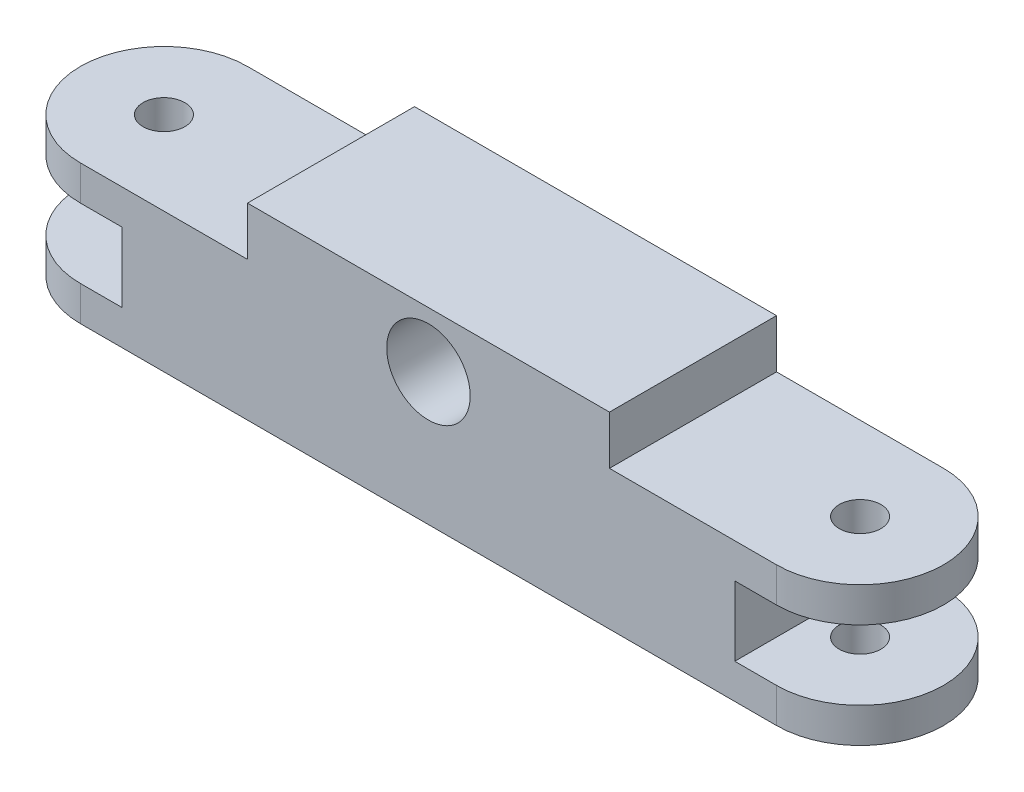
SolidWorks part; units mm, degrees
material "Plain carbon steel"
ref_plane "Front Plane" through (0, 0, 0) normal (0, 0, 1) x (1, 0, 0)
ref_plane "Top Plane" through (0, 0, 0) normal (0, 1, 0) x (1, 0, 0)
ref_plane "Right Plane" through (0, 0, 0) normal (1, 0, 0) x (0, 0, -1)
sketch "Sketch1" plane through (0, 0, 0) normal (0, 1, 0) x (1, 0, 0)
  line L0 (0, 0) -> (12, 0) construction
  line L1 (0, 6) -> (12, 6)
  line L2 (0, -6) -> (12, -6)
  arc A1 (0, 6) -> (0, -6) centre (0, 0) ccw
  arc A2 (12, -6) -> (12, 6) centre (12, 0) ccw
  circle A3 centre (0, 0) radius 1.5
  point P3 (6, 0)
  dimension "D2" = 6
  dimension "D3" = 3
  dimension "D1" = 12
extrude "Boss-Extrude1" add sketch "Sketch1" along normal blind 10
sketch "Sketch2" plane through (0, 0, 6) normal (0, 0, 1) x (1, 0, 0)
  line L0 (-6, 10) -> (-6, 0) construction
  line L1 (-6, 7.5) -> (3, 7.5)
  line L2 (-6, 7.5) -> (-6, 2.5)
  line L3 (-6, 2.5) -> (3, 2.5)
  line L4 (3, 7.5) -> (3, 2.5)
  line L5 (6, 0) -> (6, 12.6493) construction
  line L6 (0, 0) -> (12, 0) construction
  line L7 (18, 5) -> (8.4147, 5) construction
  line L8 (18, 0) -> (18, 10) construction
  line L9 (18, 7.5) -> (18, 2.5)
  line L10 (18, 2.5) -> (9, 2.5)
  line L11 (9, 7.5) -> (9, 2.5)
  line L12 (18, 7.5) -> (9, 7.5)
  dimension "D1" = 9
  dimension "D2" = 5
extrude "Cut-Extrude1" cut sketch "Sketch2" against normal through all
sketch "Sketch3" plane through (9, 0, 0) normal (1, 0, 0) x (0, 0, -1)
  line L4 (-6, 7.5) -> (-6, 2.5)
  line L5 (-6, 2.5) -> (6, 2.5)
  line L6 (6, 2.5) -> (6, 7.5)
  line L7 (6, 7.5) -> (-6, 7.5)
  line L8 (-6, 7.5) -> (-6, 2.5)
  line L9 (-6, 2.5) -> (6, 2.5)
  line L10 (6, 2.5) -> (6, 7.5)
  line L11 (6, 7.5) -> (-6, 7.5)
  dimension "D1" = 0
extrude "Boss-Extrude2" add sketch "Sketch3" along normal blind 32
ref_plane "Plane1" through (25, 0, 0) normal (1, 0, 0) x (0, 0, -1)
mirror "Mirror1" about plane through (25, 0, 0) normal (1, 0, 0) of bodies 103
sketch "Sketch5" plane through (0, 0, 6) normal (0, 0, 1) x (1, 0, 0)
  line L0 (38, 7.5) -> (12, 7.5) construction
  line L1 (12, 7.5) -> (38, 7.5)
  line L2 (12, 7.5) -> (12, 13.5)
  line L3 (12, 13.5) -> (38, 13.5)
  line L4 (38, 7.5) -> (38, 13.5)
  line L5 (12, 10) -> (12, 7.5) construction
  line L6 (38, 10) -> (38, 7.5) construction
  line L8 (12, 2.5) -> (38, 2.5)
  line L9 (12, 2.5) -> (12, 0)
  line L10 (12, 0) -> (38, 0)
  line L11 (38, 2.5) -> (38, 0)
  dimension "D1" = 0
  dimension "D2" = 0
  dimension "D3" = 6
extrude "Boss-Extrude6" add sketch "Sketch5" against normal up to surface (12 mm away) up to face at (25, 5, -6)
sketch "Sketch6" plane through (0, 0, 6) normal (0, 0, 1) x (1, 0, 0)
  line L0 (25, -55) -> (25, 55) construction
  line L2 (38, 13.5) -> (12, 13.5) construction
  circle A0 centre (25, 9.5) radius 3
  dimension "D1" = 1
  dimension "D2" = 6
extrude "Cut-Extrude2" cut sketch "Sketch6" against normal through all
